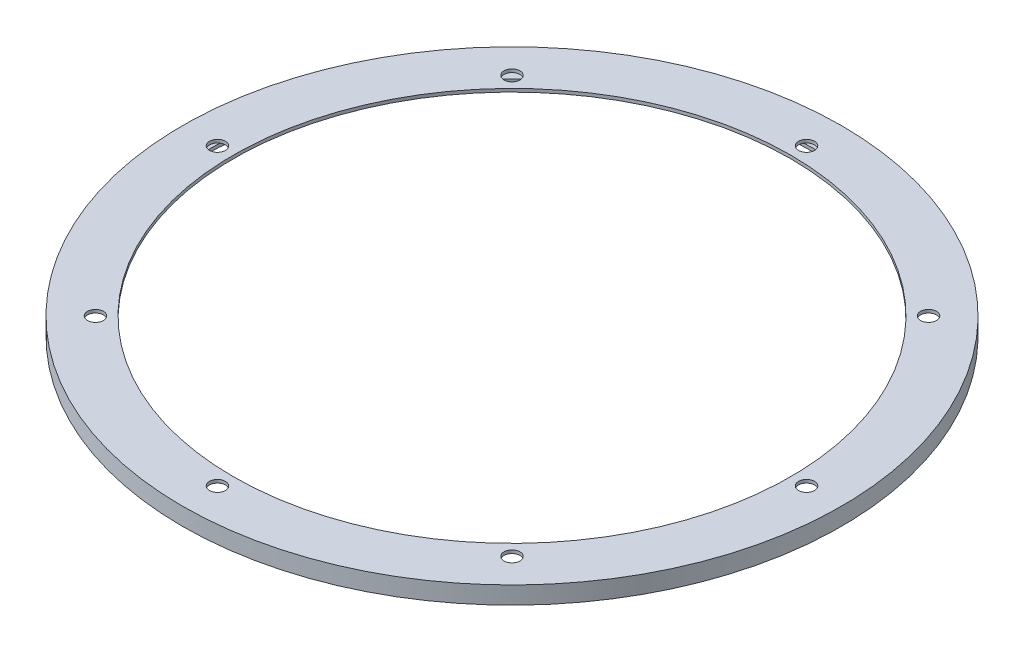
from build123d import *

# Parameters (mm, degrees)
SKETCH1_R                = 205
SKETCH1_R_2              = 5
SKETCH1_R_3              = 175
BOSS_EXTRUDE1_DEPTH      = 2
BOSS_EXTRUDE2_DEPTH      = 7
BOSS_EXTRUDE2_DEPTH_BACK = 2
SKETCH2_R                = 207
SKETCH2_R_2              = 205
BOSS_EXTRUDE3_START      = 2
SKETCH3_R                = 207
SKETCH3_R_2              = 195
BOSS_EXTRUDE3_DEPTH      = 2


with BuildPart() as part:
    # Sketch1 → Boss-Extrude1 (new body)
    with BuildSketch(Plane(origin=(0, 0, 0), x_dir=(1, 0, 0), z_dir=(0, 1, 0))):
        with Locations(Location((0, 0, 0), (0, 0, 270))):
            Circle(SKETCH1_R)
        with Locations(Location((-185, 0, 0), (0, 0, 270))):
            Circle(SKETCH1_R_2, mode=Mode.SUBTRACT)
        with Locations(Location((0, 0, 0), (0, 0, 270))):
            Circle(SKETCH1_R_3, mode=Mode.SUBTRACT)
        with Locations(Location((-130.81475452, 130.81475452, 0), (0, 0, 270))):
            Circle(SKETCH1_R_2, mode=Mode.SUBTRACT)
        with Locations(Location((0, 185, 0), (0, 0, 270))):
            Circle(SKETCH1_R_2, mode=Mode.SUBTRACT)
        with Locations(Location((130.81475452, 130.81475452, 0), (0, 0, 270))):
            Circle(SKETCH1_R_2, mode=Mode.SUBTRACT)
        with Locations(Location((185, 0, 0), (0, 0, 270))):
            Circle(SKETCH1_R_2, mode=Mode.SUBTRACT)
        with Locations(Location((130.81475452, -130.81475452, 0), (0, 0, 270))):
            Circle(SKETCH1_R_2, mode=Mode.SUBTRACT)
        with Locations(Location((0, -185, 0), (0, 0, 270))):
            Circle(SKETCH1_R_2, mode=Mode.SUBTRACT)
        with Locations(Location((-130.81475452, -130.81475452, 0), (0, 0, 270))):
            Circle(SKETCH1_R_2, mode=Mode.SUBTRACT)
    extrude(amount=BOSS_EXTRUDE1_DEPTH)

    # Sketch2 → Boss-Extrude2 (add, two sides: drawn at the far end of the back side and taken through both)
    with BuildSketch(Plane.XZ.offset(-BOSS_EXTRUDE2_DEPTH_BACK)):
        with Locations(Location((0, 0, 0), (0, 0, 270))):
            Circle(SKETCH2_R)
        with Locations(Location((0, 0, 0), (0, 0, 270))):
            Circle(SKETCH2_R_2, mode=Mode.SUBTRACT)
    extrude(amount=BOSS_EXTRUDE2_DEPTH + BOSS_EXTRUDE2_DEPTH_BACK)

    # Sketch3 → Boss-Extrude3 (add)
    with BuildSketch(Plane.XZ.offset(7).offset(BOSS_EXTRUDE3_START)):
        with Locations(Location((0, 0, 0), (0, 0, 270))):
            Circle(SKETCH3_R)
        with Locations(Location((0, 0, 0), (0, 0, 270))):
            Circle(SKETCH3_R_2, mode=Mode.SUBTRACT)
    extrude(amount=-BOSS_EXTRUDE3_DEPTH)


solid = part.part
